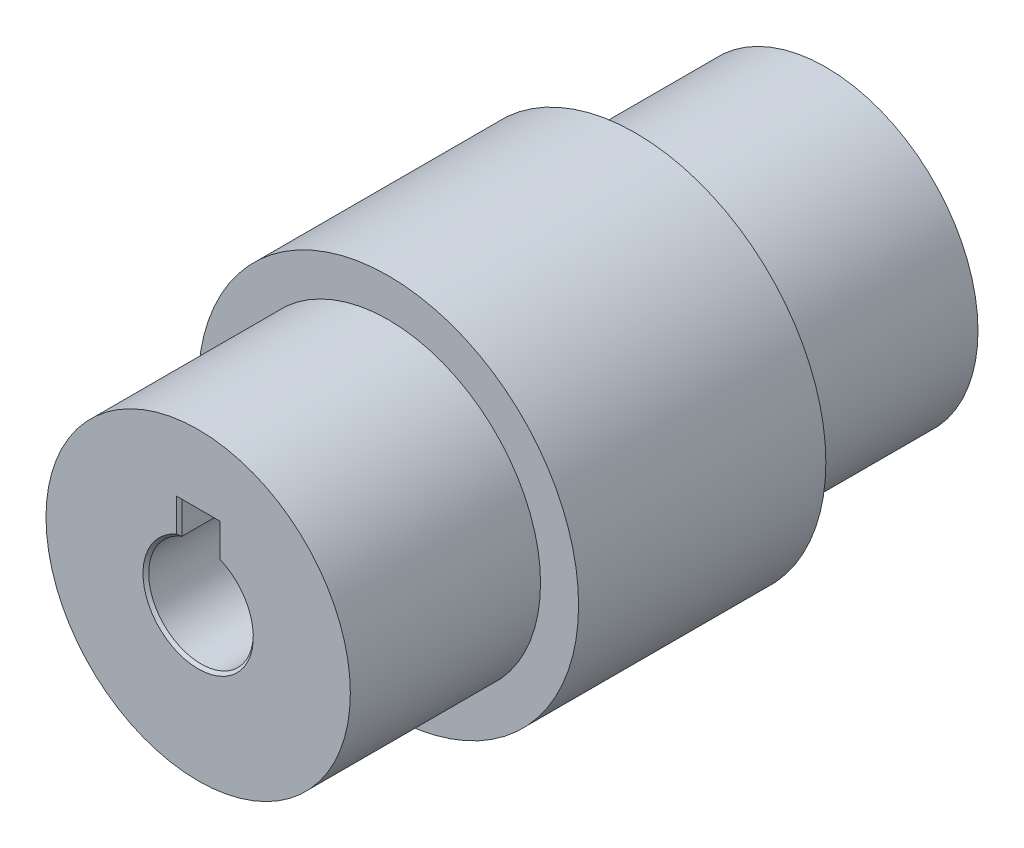
from build123d import *

# Parameters (mm, degrees)
SKETCH_1_R          = 16
EXTRUDE_1_DEPTH     = 20
SKETCH_2_R          = 20
EXTRUDE_2_DEPTH     = 26
SKETCH_3_R          = 16
EXTRUDE_3_DEPTH     = 20
SKETCH_4_R          = 9.5
CUT_EXTRUDE_1_DEPTH = 27
SKETCH_5_R          = 5.5
CUT_EXTRUDE_2_DEPTH = 27
SKETCH_6_R          = 10
CUT_EXTRUDE_3_DEPTH = 12
CUT_EXTRUDE_4_DEPTH = 27
CUT_EXTRUDE_5_DEPTH = 27
CHAMFER_1_SIZE      = 0.3


with BuildPart() as part:
    # 草图1 → 拉伸1 (new body)
    with BuildSketch(Plane(origin=(0, 0, 0), x_dir=(0, -1, 0), z_dir=(0, 0, 1))):
        with Locations(Location((0, 0, 0), (0, 0, 90))):
            Circle(SKETCH_1_R)
    extrude(amount=EXTRUDE_1_DEPTH)

    # 草图2 → 拉伸2 (add)
    with BuildSketch(Plane(origin=(0, 0, 20), x_dir=(0, 1, 0), z_dir=(0, 0, 1))):
        with Locations(Location((0, 0, 0), (0, 0, 90))):
            Circle(SKETCH_2_R)
    extrude(amount=EXTRUDE_2_DEPTH)

    # 草图3 → 拉伸3 (add)
    with BuildSketch(Plane(origin=(0, 0, 46), x_dir=(0, 1, 0), z_dir=(0, 0, 1))):
        with Locations(Location((0, 0, 0), (0, 0, 270))):
            Circle(SKETCH_3_R)
    extrude(amount=EXTRUDE_3_DEPTH)

    # 草图4 → 切除-拉伸1 (cut)
    with BuildSketch(Plane(origin=(0, 0, 0), x_dir=(-1, 0, 0), z_dir=(0, 0, -1))):
        Circle(SKETCH_4_R)
    extrude(amount=-CUT_EXTRUDE_1_DEPTH, mode=Mode.SUBTRACT)

    # 草图5 → 切除-拉伸2 (cut)
    with BuildSketch(Plane.XY.offset(66)):
        Circle(SKETCH_5_R)
    extrude(amount=-CUT_EXTRUDE_2_DEPTH, mode=Mode.SUBTRACT)

    # 草图6 → 切除-拉伸3 (cut)
    with BuildSketch(Plane.XY.offset(39)):
        Circle(SKETCH_6_R)
    extrude(amount=-CUT_EXTRUDE_3_DEPTH, mode=Mode.SUBTRACT)

    # 草图7 → 切除-拉伸4 (cut)
    with BuildSketch(Plane(origin=(0, 0, 0), x_dir=(-1, 0, 0), z_dir=(0, 0, -1))):
        with BuildLine():
            Line((-3, 12), (-3, 9.013878189))
            ThreePointArc((-3, 9.013878189), (0, 9.5), (3, 9.013878189))
            Line((3, 9.013878189), (3, 12))
            Line((3, 12), (-3, 12))
        make_face()
    extrude(amount=-CUT_EXTRUDE_4_DEPTH, mode=Mode.SUBTRACT)

    # 草图8 → 切除-拉伸5 (cut)
    with BuildSketch(Plane.XY.offset(66)):
        with BuildLine():
            Line((-2, 8.5), (-2, 5.123475383))
            ThreePointArc((-2, 5.123475383), (0, 5.5), (2, 5.123475383))
            Line((2, 5.123475383), (2, 8.5))
            Line((2, 8.5), (-2, 8.5))
        make_face()
    extrude(amount=-CUT_EXTRUDE_5_DEPTH, mode=Mode.SUBTRACT)

    # 倒角1
    chamfer_1_edges = [part.edges().sort_by_distance(p)[0] for p in [
        (0, -9.5, 0),
        (0, 12, 0),
        (3, 10.506939094, 0),
        (-3, 10.506939094, 0),
        (0, -5.5, 66),
        (0, 8.5, 66),
        (-2, 6.811737691, 66),
        (2, 6.811737691, 66),
    ]]
    chamfer(chamfer_1_edges, length=CHAMFER_1_SIZE)


solid = part.part
